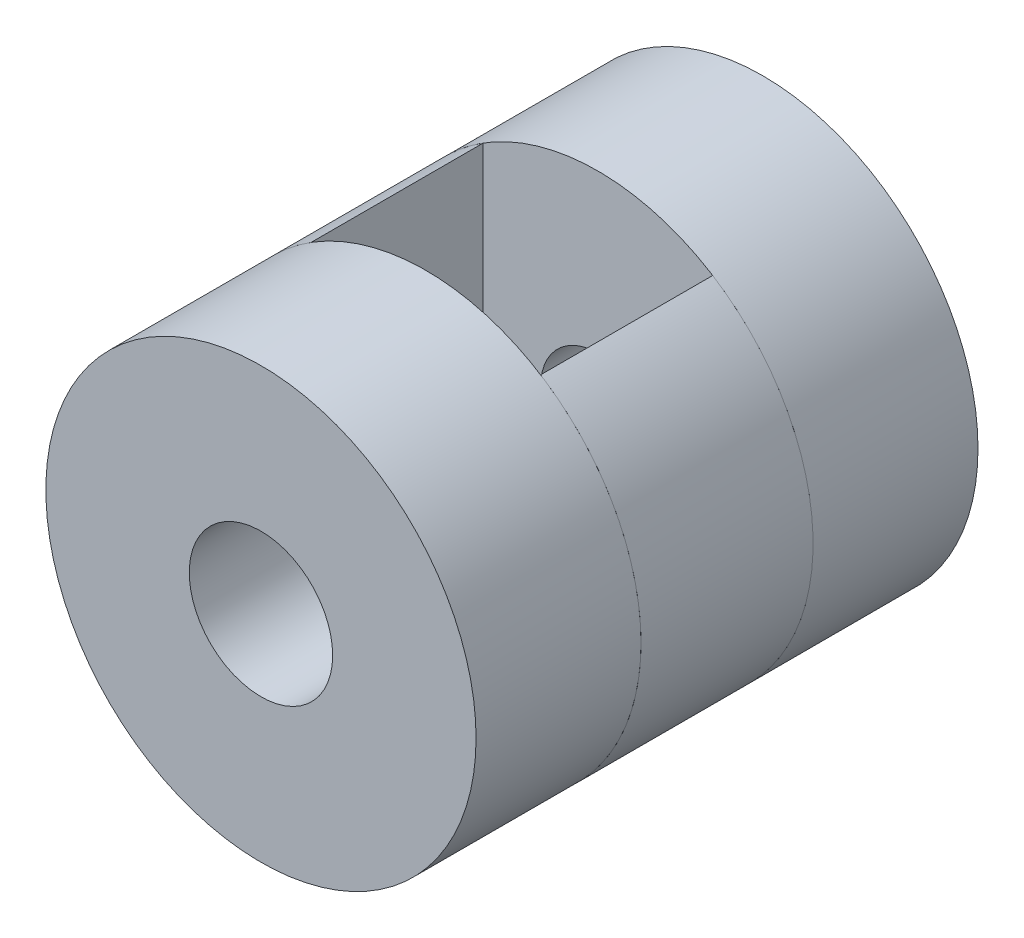
SolidWorks part; units mm, degrees
ref_plane "Front Plane" through (0, 0, 0) normal (0, 0, 1) x (1, 0, 0)
ref_plane "Top Plane" through (0, 0, 0) normal (0, 1, 0) x (1, 0, 0)
ref_plane "Right Plane" through (0, 0, 0) normal (1, 0, 0) x (0, 0, -1)
sketch "Sketch1" plane through (0, 0, 0) normal (0, 0, 1) x (1, 0, 0)
  circle A0 centre (0, 0) radius 15
  circle A1 centre (0, 0) radius 4
  dimension "D1" = 30
  dimension "D2" = 8
extrude "Boss-Extrude1" add sketch "Sketch1" along normal mid plane 35
sketch "Sketch2" plane through (0, 0, 0) normal (0, 1, 0) x (1, 0, 0)
  line L1 (-8, -6) -> (8, -6)
  line L2 (-8, -6) -> (-8, 6)
  line L3 (-8, 6) -> (8, 6)
  line L4 (8, -6) -> (8, 6)
  line L5 (-8, -6) -> (8, 6) construction
  line L6 (-8, 6) -> (8, -6) construction
  point P0 (0, 0)
  dimension "D1" = 12
  dimension "D2" = 16
extrude "Cut-Extrude1" cut sketch "Sketch2" against normal mid plane 35
sketch "Sketch3" plane through (0, 0, 17.5) normal (0, 0, 1) x (1, 0, 0)
  circle A0 centre (0, 0) radius 5
  dimension "D1" = 10
extrude "Cut-Extrude2" cut sketch "Sketch3" against normal up to next
sketch "Sketch4" plane through (0, 0, 0) normal (0, 1, 0) x (1, 0, 0)
  line L0 (15, -17.5) -> (15, 17.5) construction
  line L1 (-15, 6) -> (15, 6)
  line L2 (-15, 6) -> (-15, -6)
  line L3 (-15, -6) -> (15, -6)
  line L4 (15, 6) -> (15, -6)
  line L5 (-15, 6) -> (15, -6) construction
  line L6 (-15, -6) -> (15, 6) construction
  point P0 (0, 0)
  dimension "D1" = 12
split "Split1" trim tools "Sketch4" resulting bodies 106 107 108 109
